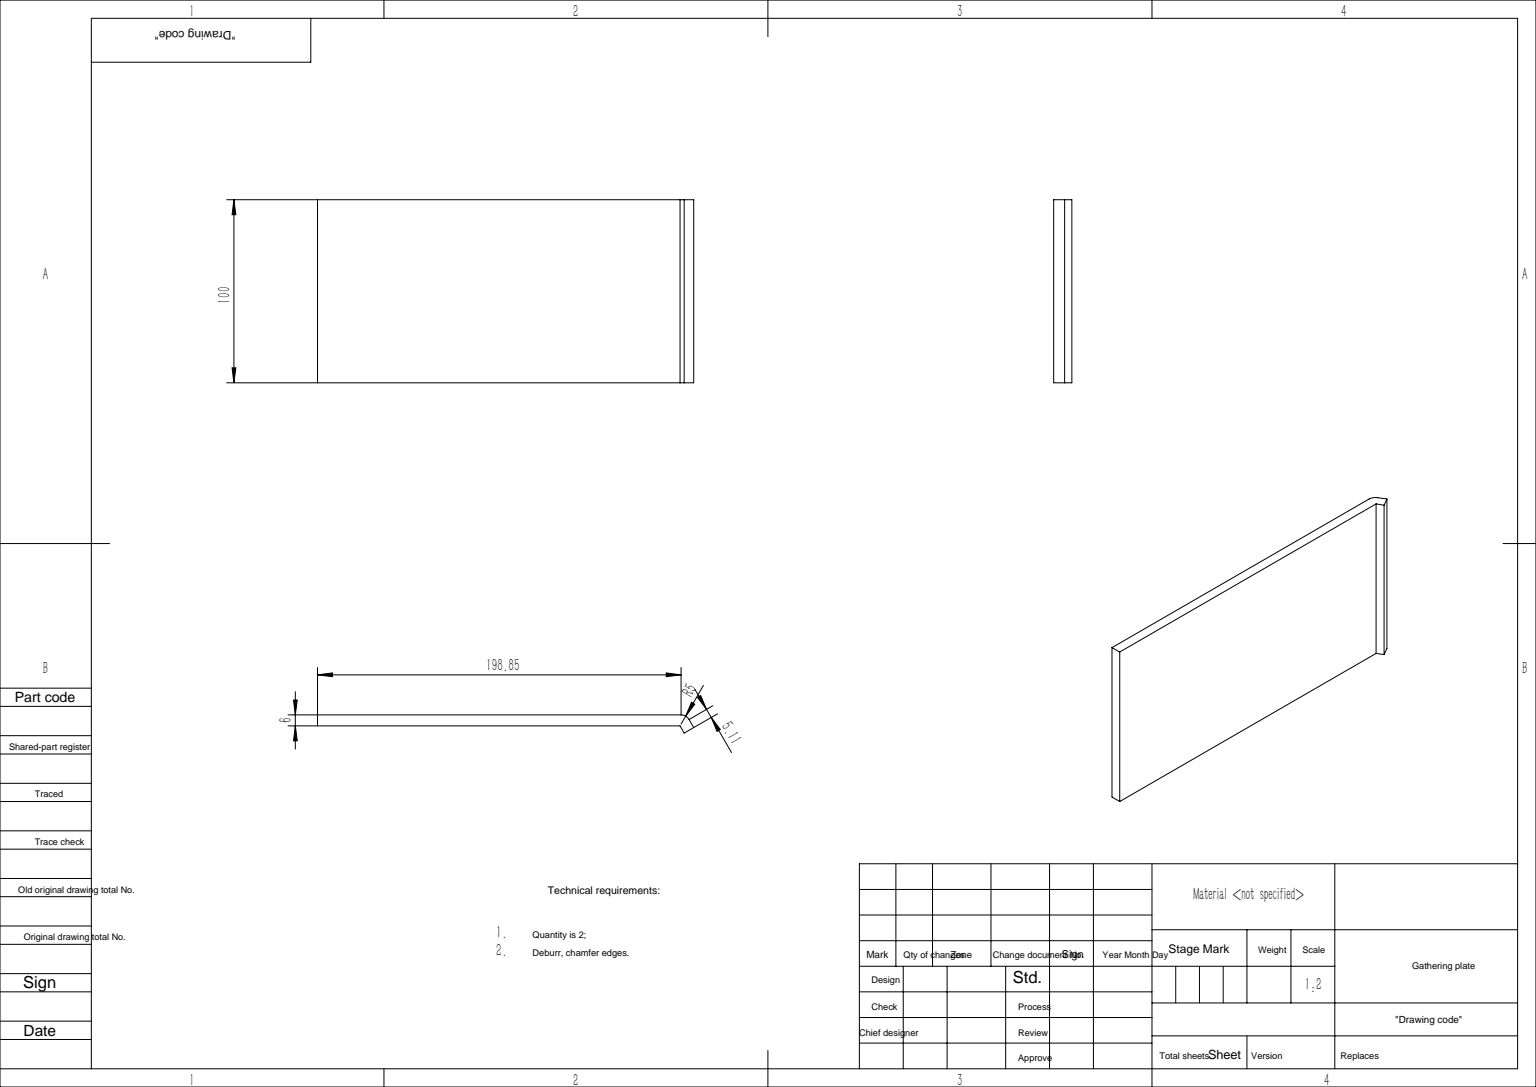
SolidWorks part; units mm, degrees
ref_plane "前视基准面" through (0, 0, 0) normal (0, 0, 1) x (1, 0, 0)
ref_plane "上视基准面" through (0, 0, 0) normal (0, 1, 0) x (1, 0, 0)
ref_plane "右视基准面" through (0, 0, 0) normal (1, 0, 0) x (0, 0, -1)
sketch "草图1" plane through (0, 0, 0) normal (0, 1, 0) x (1, 0, 0)
  line L0 (0, 0) -> (0, 200) construction
  line L1 (0, 200) -> (5, 202.8868) construction
  line L2 (3, 0) -> (3, 198.2679)
  line L3 (3, 198.2679) -> (6.9282, 200.5359)
  line L4 (-3, 0) -> (-3, 201.7321)
  line L5 (-3, 201.7321) -> (3.9282, 205.7321)
  line L6 (-3, 0) -> (3, 0)
  line L7 (3.9282, 205.7321) -> (6.9282, 200.5359)
  line L8 (0, 200) -> (5.4282, 203.134) construction
  dimension "D1" = 5
  dimension "D2" = 120
  dimension "D3" = 200
  dimension "D6" = 8
  dimension "D4" = 3
  dimension "D5" = 3
extrude "凸台-拉伸1" add sketch "草图1" along normal blind 100
fillet "圆角1" radius 5 1 edges at (-3, 50, -201.7321)
